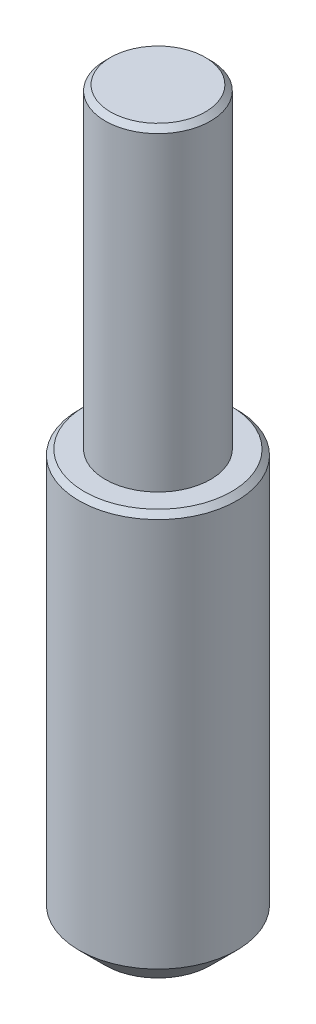
SolidWorks part; units mm, degrees
ref_plane "Front Plane" through (0, 0, 0) normal (0, 0, 1) x (1, 0, 0)
ref_plane "Top Plane" through (0, 0, 0) normal (0, 1, 0) x (1, 0, 0)
ref_plane "Right Plane" through (0, 0, 0) normal (1, 0, 0) x (0, 0, -1)
other "Configuration Table"
sketch "Sketch1" plane through (0, 0, 0) normal (0, 0, 1) x (1, 0, 0)
  line L0 (0, 13.3593) -> (0, -12.7871) construction
  line L1 (0, 0) -> (-2, 0)
  line L2 (-3, 1) -> (-3, 15.8)
  line L3 (-2.8, 16) -> (-2, 16)
  line L4 (-2, 16) -> (-2, 27.8)
  line L5 (-1.8, 28) -> (0, 28)
  line L6 (0, 28) -> (0, 0)
  line L7 (-2, 0) -> (-3, 1)
  line L8 (-2, 27.8) -> (-1.8, 28)
  line L9 (-3, 15.8) -> (-2.8, 16)
  point P4 (-3, 0)
  point P6 (-3, 16)
  point P8 (-2, 28)
  dimension "D1" = 16
  dimension "D2" = 28
  dimension "D3" = 2
  dimension "D4" = 3
  dimension "D5" = 1
  dimension "D6" = 45
  dimension "D7" = 0.2
  dimension "D8" = 45
  dimension "D9" = 0.2
  dimension "D10" = 45
revolve "Revolve1" add sketch "Sketch1" angle 360 about L0
